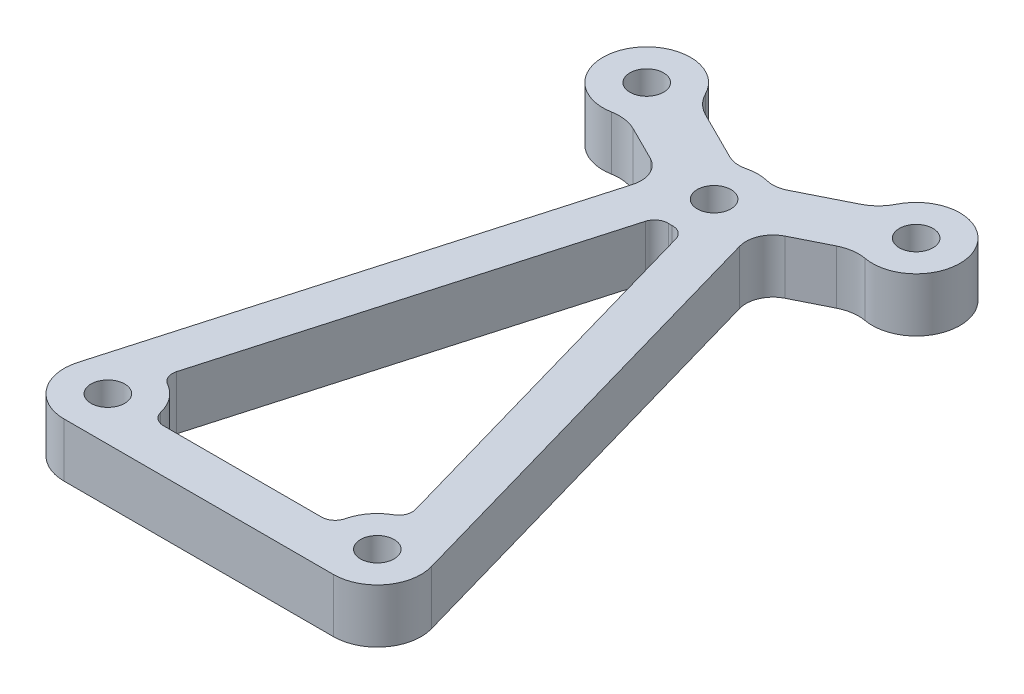
from build123d import *

# Parameters (mm, degrees)
SKETCH_1_R      = 3.25
SKETCH_1_R_2    = 1.25
EXTRUDE_1_DEPTH = 4
FILLET_1_R      = 1
FILLET_2_R      = 2
FILLET_3_R      = 3


with BuildPart() as part:
    # 草图1 → 凸台-拉伸1 (new body)
    # profile 1 of 12: a face of its own
    with BuildSketch(Plane(origin=(0, 0, 0), x_dir=(1, 0, 0), z_dir=(0, 1, 0))):
        with Locations((-10, 40)):
            Circle(SKETCH_1_R)
        with Locations(Location((-10, 40, 0), (0, 0, 270))):
            Circle(SKETCH_1_R_2, mode=Mode.SUBTRACT)
    # profile 2 of 12: a face of its own
    with BuildSketch(Plane(origin=(0, 0, 0), x_dir=(1, 0, 0), z_dir=(0, 1, 0))):
        with BuildLine():
            Line((-8.603139344, 37.065501694), (-3.516561637, 34.522212841))
            Line((-3.516561637, 34.522212841), (-3.12495283, 35.892843666))
            ThreePointArc((-3.12495283, 35.892843666), (-2.480682914, 37.099693378), (-1.396860656, 37.934498306))
            Line((-1.396860656, 37.934498306), (-6.814284962, 40.643210458))
            ThreePointArc((-6.814284962, 40.643210458), (-6.766111174, 40.32320746), (-6.75, 40))
            ThreePointArc((-6.75, 40), (-7.252064672, 38.26467541), (-8.603139344, 37.065501694))
        make_face()
    # profile 3 of 12: a face of its own
    with BuildSketch(Plane(origin=(0, 0, 0), x_dir=(1, 0, 0), z_dir=(0, 1, 0))):
        with BuildLine():
            ThreePointArc((-13.12495283, 0.892843666), (-11.578339526, 2.841011147), (-9.107156334, 3.12495283))
            Line((-9.107156334, 3.12495283), (-0.892843666, 31.87504717))
            ThreePointArc((-0.892843666, 31.87504717), (-2.38713669, 32.79453442), (-3.185715038, 34.356789542))
            Line((-3.185715038, 34.356789542), (-3.516561637, 34.522212841))
            Line((-3.516561637, 34.522212841), (-13.12495283, 0.892843666))
        make_face()
    # profile 4 of 12: a face of its own
    with BuildSketch(Plane(origin=(0, 0, 0), x_dir=(1, 0, 0), z_dir=(0, 1, 0))):
        with BuildLine():
            ThreePointArc((3.185715038, 34.356789542), (2.38713669, 32.79453442), (0.892843666, 31.87504717))
            Line((0.892843666, 31.87504717), (9.107156334, 3.12495283))
            ThreePointArc((9.107156334, 3.12495283), (11.578339526, 2.841011147), (13.12495283, 0.892843666))
            Line((13.12495283, 0.892843666), (3.516561637, 34.522212841))
            Line((3.516561637, 34.522212841), (3.185715038, 34.356789542))
        make_face()
    # profile 5 of 12: a face of its own
    with BuildSketch(Plane(origin=(0, 0, 0), x_dir=(1, 0, 0), z_dir=(0, 1, 0))):
        with Locations((-10, 0)):
            Circle(SKETCH_1_R)
        with Locations(Location((-10, 0, 0), (0, 0, 270))):
            Circle(SKETCH_1_R_2, mode=Mode.SUBTRACT)
    # profile 6 of 12: a face of its own
    with BuildSketch(Plane(origin=(0, 0, 0), x_dir=(1, 0, 0), z_dir=(0, 1, 0))):
        with BuildLine():
            Line((6.75, 0), (-6.75, 0))
            ThreePointArc((-6.75, 0), (-7.701902961, -2.298097039), (-10, -3.25))
            Line((-10, -3.25), (10, -3.25))
            ThreePointArc((10, -3.25), (7.701902961, -2.298097039), (6.75, 0))
        make_face()
    # profile 7 of 12: a face of its own
    with BuildSketch(Plane(origin=(0, 0, 0), x_dir=(1, 0, 0), z_dir=(0, 1, 0))):
        with Locations((10, 0)):
            Circle(SKETCH_1_R)
        with Locations(Location((10, 0, 0), (0, 0, 270))):
            Circle(SKETCH_1_R_2, mode=Mode.SUBTRACT)
    # profile 8 of 12: a face of its own
    with BuildSketch(Plane(origin=(0, 0, 0), x_dir=(1, 0, 0), z_dir=(0, 1, 0))):
        with Locations((0, 35)):
            Circle(SKETCH_1_R)
        with Locations(Location((0, 35, 0), (0, 0, 270))):
            Circle(SKETCH_1_R_2, mode=Mode.SUBTRACT)
    # profile 9 of 12: a face of its own
    with BuildSketch(Plane(origin=(0, 0, 0), x_dir=(1, 0, 0), z_dir=(0, 1, 0))):
        with BuildLine():
            Line((-3.516561637, 34.522212841), (-3.185715038, 34.356789542))
            ThreePointArc((-3.185715038, 34.356789542), (-3.247460208, 35.128460874), (-3.12495283, 35.892843666))
            Line((-3.12495283, 35.892843666), (-3.516561637, 34.522212841))
        make_face()
    # profile 10 of 12: a face of its own
    with BuildSketch(Plane(origin=(0, 0, 0), x_dir=(1, 0, 0), z_dir=(0, 1, 0))):
        with BuildLine():
            ThreePointArc((3.25, 35), (3.233888826, 34.67679254), (3.185715038, 34.356789542))
            Line((3.185715038, 34.356789542), (3.516561637, 34.522212841))
            Line((3.516561637, 34.522212841), (3.12495283, 35.892843666))
            ThreePointArc((3.12495283, 35.892843666), (3.21858639, 35.450778939), (3.25, 35))
        make_face()
    # profile 11 of 12: a face of its own
    with BuildSketch(Plane(origin=(0, 0, 0), x_dir=(1, 0, 0), z_dir=(0, 1, 0))):
        with BuildLine():
            Line((3.12495283, 35.892843666), (3.516561637, 34.522212841))
            Line((3.516561637, 34.522212841), (8.603139344, 37.065501694))
            ThreePointArc((8.603139344, 37.065501694), (7.093111629, 38.546555815), (6.814284962, 40.643210458))
            Line((6.814284962, 40.643210458), (1.396860656, 37.934498306))
            ThreePointArc((1.396860656, 37.934498306), (2.480682914, 37.099693378), (3.12495283, 35.892843666))
        make_face()
    # profile 12 of 12: a face of its own
    with BuildSketch(Plane(origin=(0, 0, 0), x_dir=(1, 0, 0), z_dir=(0, 1, 0))):
        with Locations((10, 40)):
            Circle(SKETCH_1_R)
        with Locations(Location((10, 40, 0), (0, 0, 270))):
            Circle(SKETCH_1_R_2, mode=Mode.SUBTRACT)
    extrude(amount=EXTRUDE_1_DEPTH)

    # 圆角1
    fillet_1_edges = [part.edges().sort_by_distance(p)[0] for p in [
        (9.107156334, 2, -3.12495283),
        (0.892843666, 2, -31.87504717),
        (-0.892843666, 2, -31.87504717),
        (-9.107156334, 2, -3.12495283),
        (-6.75, 2, 0),
        (6.75, 2, 0),
    ]]
    fillet(fillet_1_edges, radius=FILLET_1_R)

    # 圆角2
    fillet_2_edges = [part.edges().sort_by_distance(p)[0] for p in [
        (-3.516561637, 2, -34.522212841),
        (-1.396860656, 2, -37.934498306),
        (1.396860656, 2, -37.934498306),
        (3.516561637, 2, -34.522212841),
    ]]
    fillet(fillet_2_edges, radius=FILLET_2_R)

    # 圆角3
    fillet_3_edges = [part.edges().sort_by_distance(p)[0] for p in [
        (-8.603139344, 2, -37.065501694),
        (-6.814284962, 2, -40.643210458),
        (6.814284962, 2, -40.643210458),
        (8.603139344, 2, -37.065501694),
    ]]
    fillet(fillet_3_edges, radius=FILLET_3_R)


solid = part.part
